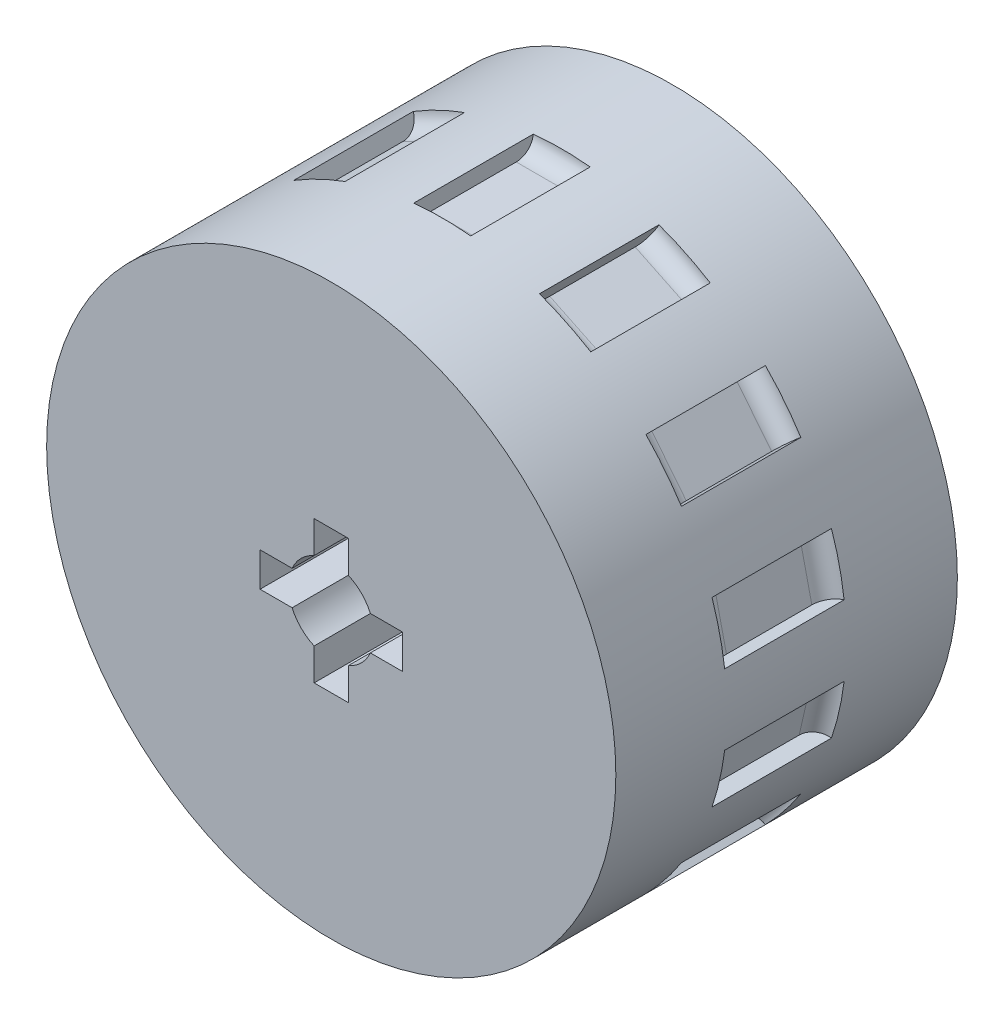
SolidWorks part; units mm, degrees
ref_plane "前视基准面" through (0, 0, 0) normal (0, 0, 1) x (1, 0, 0)
ref_plane "上视基准面" through (0, 0, 0) normal (0, 1, 0) x (1, 0, 0)
ref_plane "右视基准面" through (0, 0, 0) normal (1, 0, 0) x (0, 0, -1)
sketch "草图1" plane through (0, 0, 0) normal (0, 0, 1) x (1, 0, 0)
  line L2 (3, -6.8739) -> (3, -12.5)
  line L3 (-3, 12.5) -> (3, 12.5)
  line L4 (-3, 12.5) -> (-3, 6.8739)
  line L5 (-3, -12.5) -> (3, -12.5)
  line L6 (3, 12.5) -> (3, 6.8739)
  line L7 (-12.5, -3) -> (-6.8739, -3)
  line L8 (-12.5, -3) -> (-12.5, 3)
  line L9 (-12.5, 3) -> (-6.8739, 3)
  line L10 (12.5, -3) -> (12.5, 3)
  line L11 (-3, -6.8739) -> (-3, -12.5)
  line L12 (6.8739, 3) -> (12.5, 3)
  line L13 (6.8739, -3) -> (12.5, -3)
  line L14 (0, 12.5) -> (0, -12.5) construction
  line L15 (-12.5, 0) -> (12.5, 0) construction
  circle A0 centre (0, 0) radius 50
  arc A1 (-3, 6.8739) -> (-6.8739, 3) centre (0, 0) ccw
  arc A2 (-6.8739, -3) -> (-3, -6.8739) centre (0, 0) ccw
  arc A3 (6.8739, 3) -> (3, 6.8739) centre (0, 0) ccw
  arc A7 (3, -6.8739) -> (6.8739, -3) centre (0, 0) ccw
  dimension "D1" = 100
  dimension "D2" = 25
  dimension "D4" = 25
  dimension "D6" = 6
  dimension "D9" = 6
extrude "拉伸1" add sketch "草图1" along normal blind 60
sketch "草图2" plane through (0, 0, 0) normal (0, 0, -1) x (-1, 0, 0)
  circle A0 centre (0, 0) radius 13
  circle A1 centre (0, 0) radius 7.5
  dimension "D1" = 26
  dimension "D2" = 15
extrude "凸台-拉伸1" add sketch "草图2" along normal blind 5
sketch "草图3" plane through (0, 0, 0) normal (1, 0, 0) x (0, 0, -1)
  line L0 (-37.5, 50) -> (-22.5, 50) construction
  line L3 (0, 50) -> (-60, 50) construction
  line L4 (-37.5, 53) -> (-22.5, 53)
  line L5 (-37.5, 47) -> (-22.5, 47)
  arc A4 (-37.5, 53) -> (-37.5, 47) centre (-37.5, 50) ccw
  arc A5 (-22.5, 47) -> (-22.5, 53) centre (-22.5, 50) ccw
  point P7 (-30, 50)
  dimension "D1" = 6
  dimension "D2" = 15
extrude "切除-拉伸1" cut sketch "草图3" against normal mid plane 10
pattern_circular "阵列(圆周)1" count 14 over 360 about axis through (0, 0, 0) along (0, 0, 1) of "切除-拉伸1"
